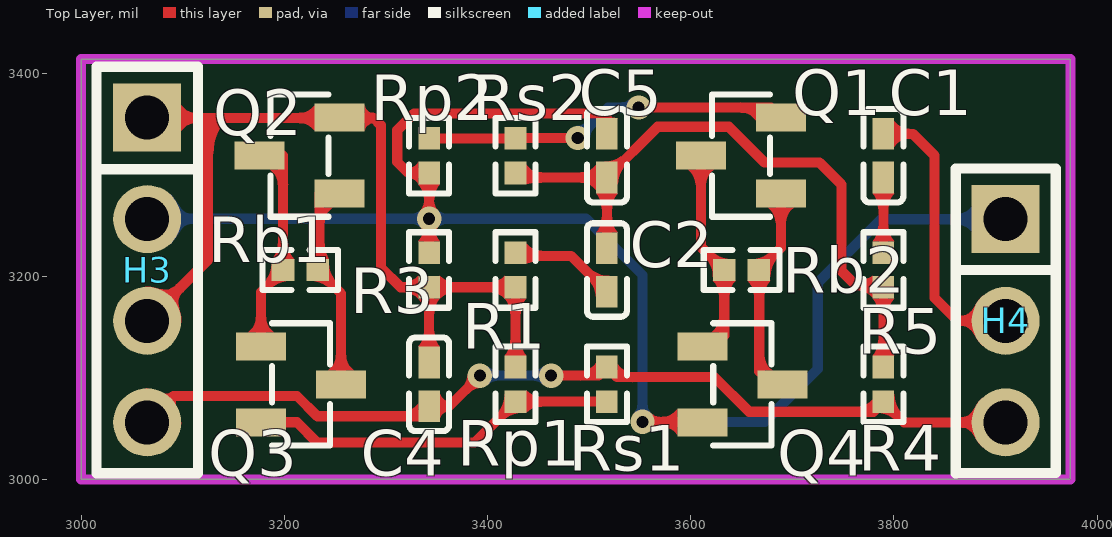
[diagram p0: Top Layer view]
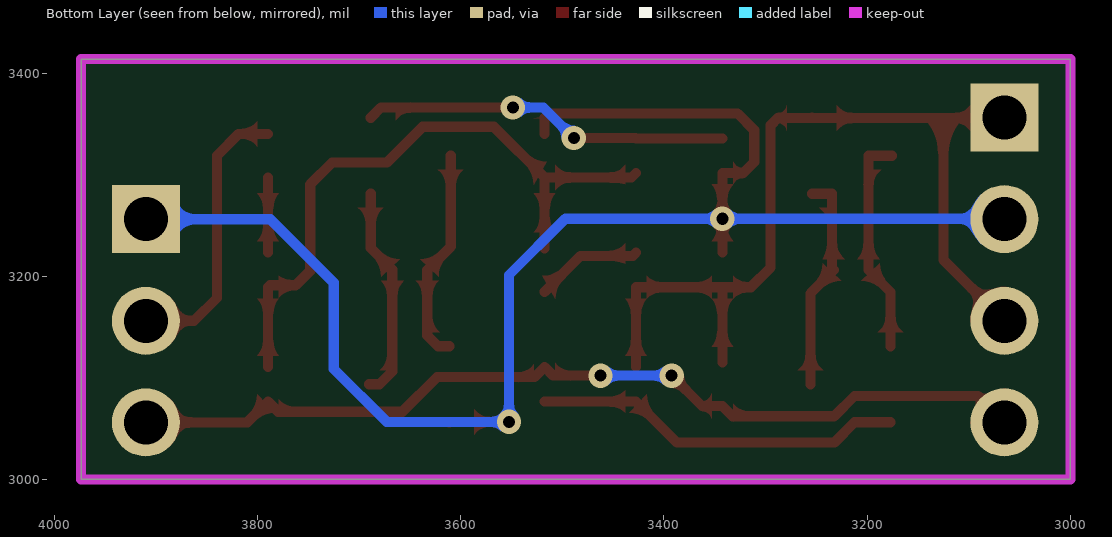
[diagram p1: Bottom Layer view, seen from below]
# Altium PCB MISC51661.pcbdoc
Units mil, origin at the board's own origin, x right, y up, seen from the top; angles counter-clockwise.
Board outline 973.64 x 413.7 mil, 2 copper layers (Top Layer, Bottom Layer), stack 62.206 mil thick; 20 components, 13 nets, 47 pads, 6 vias.

## Layer stack, top to bottom
Top Solder Mask Layer: solder mask 0.394, Dk 3.3
Top Layer: signal copper 1.379
Dielectric1: surface 59.449, FR4, Dk 4.5
Bottom Layer: signal copper 1.378
Bottom Solder Mask Layer: solder mask 0.394, Dk 3.3

## Board outline
3000,3413.7 3000,3000 3973.64,3000 3973.64,3413.7

## Design rules (kind name [scope] priority, off if disabled: settings)
BoardOutlineClearance copperThickness2oz_1 [All] p2 off: genericclearance=7.99 ignorepadtopadclearanceinfootprint=FALSE except(0: Arc-SplitContinuation Track-SplitContinuation SMDPad-SplitContinuation THPad-SplitContinuation Via-SplitContinuation Fill-SplitContinuation Region-SplitContinuation Poly-SplitContinuation Text-SplitContinuation Hole-SplitContinuation; 5.98: Arc-CutoutEdge Track-CutoutEdge SMDPad-CutoutEdge THPad-CutoutEdge Via-CutoutEdge Text-CutoutEdge; 6.9: Hole-OutlineEdge Hole-CutoutEdge; 10: Poly-OutlineEdge Poly-CutoutEdge; 11.81: Arc-OutlineEdge Track-OutlineEdge SMDPad-OutlineEdge THPad-OutlineEdge Via-OutlineEdge Fill-OutlineEdge Region-OutlineEdge Text-OutlineEdge Fill-CutoutEdge Region-CutoutEdge)
BoardOutlineClearance Plane_innerPlane_1 [All] p4 off: genericclearance=4.02 ignorepadtopadclearanceinfootprint=FALSE except(0: Arc-SplitContinuation Track-SplitContinuation SMDPad-SplitContinuation THPad-SplitContinuation Via-SplitContinuation Fill-SplitContinuation Region-SplitContinuation Poly-SplitContinuation Text-SplitContinuation Hole-SplitContinuation; 5.98: Arc-CutoutEdge Track-CutoutEdge SMDPad-CutoutEdge THPad-CutoutEdge Via-CutoutEdge Text-CutoutEdge; 6.9: Hole-OutlineEdge Hole-CutoutEdge; 10: Poly-OutlineEdge Poly-CutoutEdge; 11.81: Arc-OutlineEdge Track-OutlineEdge SMDPad-OutlineEdge THPad-OutlineEdge Via-OutlineEdge Fill-OutlineEdge Region-OutlineEdge Text-OutlineEdge Fill-CutoutEdge Region-CutoutEdge)
BoardOutlineClearance Copper_copperRegion_1 [All] p6 off: genericclearance=4.02 ignorepadtopadclearanceinfootprint=FALSE except(0: Arc-SplitContinuation Track-SplitContinuation SMDPad-SplitContinuation THPad-SplitContinuation Via-SplitContinuation Fill-SplitContinuation Region-SplitContinuation Poly-SplitContinuation Text-SplitContinuation Hole-SplitContinuation; 5.98: Arc-CutoutEdge Track-CutoutEdge SMDPad-CutoutEdge THPad-CutoutEdge Via-CutoutEdge Text-CutoutEdge; 6.9: Hole-OutlineEdge Hole-CutoutEdge; 10: Poly-OutlineEdge Poly-CutoutEdge; 11.81: Arc-OutlineEdge Track-OutlineEdge SMDPad-OutlineEdge THPad-OutlineEdge Via-OutlineEdge Fill-OutlineEdge Region-OutlineEdge Text-OutlineEdge Fill-CutoutEdge Region-CutoutEdge)
BoardOutlineClearance copperThickness1oz_1 [All] p8: genericclearance=4.02 ignorepadtopadclearanceinfootprint=FALSE except(0: Arc-SplitContinuation Track-SplitContinuation SMDPad-SplitContinuation THPad-SplitContinuation Via-SplitContinuation Fill-SplitContinuation Region-SplitContinuation Poly-SplitContinuation Text-SplitContinuation Hole-SplitContinuation; 5.98: Arc-CutoutEdge Track-CutoutEdge SMDPad-CutoutEdge THPad-CutoutEdge Via-CutoutEdge Text-CutoutEdge; 6.9: Hole-OutlineEdge Hole-CutoutEdge; 10: Poly-OutlineEdge Poly-CutoutEdge; 11.81: Arc-OutlineEdge Track-OutlineEdge SMDPad-OutlineEdge THPad-OutlineEdge Via-OutlineEdge Fill-OutlineEdge Region-OutlineEdge Text-OutlineEdge Fill-CutoutEdge Region-CutoutEdge)
Clearance copperThickness2oz [All] p1 off: gap=7.99 ignorepadtopadclearanceinfootprint=FALSE except(5.98: SMDPad-Track SMDPad-SMDPad THPad-Track SMDPad-THPad THPad-THPad Track-Via SMDPad-Via THPad-Via Via-Via Fill-SMDPad Region-SMDPad Fill-THPad Region-THPad Fill-Via Region-Via Fill-Fill Fill-Region Region-Region Arc-Track Arc-SMDPad Arc-THPad Arc-Via Fill-Arc Region-Arc Arc-Arc Text-Track SMDPad-Text Text-THPad Text-Via Fill-Text Region-Text Arc-Text Text-Text; 6.9: Hole-Track Hole-SMDPad Hole-THPad Hole-Via Fill-Hole Region-Hole Hole-Arc Hole-Text; 10: Poly-Track Poly-SMDPad Poly-THPad Poly-Via Poly-Fill Poly-Region Poly-Poly Poly-Arc Poly-Text Poly-Hole; 11.81: Fill-Track Region-Track)
Clearance Plane_innerPlane [All] p3 off: gap=4.02 ignorepadtopadclearanceinfootprint=FALSE except(5.98: SMDPad-Track SMDPad-SMDPad THPad-Track SMDPad-THPad THPad-THPad Track-Via SMDPad-Via THPad-Via Via-Via Fill-SMDPad Region-SMDPad Fill-THPad Region-THPad Fill-Via Region-Via Fill-Fill Fill-Region Region-Region Arc-Track Arc-SMDPad Arc-THPad Arc-Via Fill-Arc Region-Arc Arc-Arc Text-Track SMDPad-Text Text-THPad Text-Via Fill-Text Region-Text Arc-Text Text-Text; 6.9: Hole-Track Hole-SMDPad Hole-THPad Hole-Via Fill-Hole Region-Hole Hole-Arc Hole-Text; 10: Poly-Track Poly-SMDPad Poly-THPad Poly-Via Poly-Fill Poly-Region Poly-Poly Poly-Arc Poly-Text Poly-Hole; 11.81: Fill-Track Region-Track)
Clearance Copper_copperRegion [All] p5 off: gap=4.02 ignorepadtopadclearanceinfootprint=FALSE except(5.98: SMDPad-Track SMDPad-SMDPad THPad-Track SMDPad-THPad THPad-THPad Track-Via SMDPad-Via THPad-Via Via-Via Fill-SMDPad Region-SMDPad Fill-THPad Region-THPad Fill-Via Region-Via Fill-Fill Fill-Region Region-Region Arc-Track Arc-SMDPad Arc-THPad Arc-Via Fill-Arc Region-Arc Arc-Arc Text-Track SMDPad-Text Text-THPad Text-Via Fill-Text Region-Text Arc-Text Text-Text; 6.9: Hole-Track Hole-SMDPad Hole-THPad Hole-Via Fill-Hole Region-Hole Hole-Arc Hole-Text; 10: Poly-Track Poly-SMDPad Poly-THPad Poly-Via Poly-Fill Poly-Region Poly-Poly Poly-Arc Poly-Text Poly-Hole; 11.81: Fill-Track Region-Track)
Clearance copperThickness1oz [All] p7: gap=4.02 ignorepadtopadclearanceinfootprint=FALSE except(5.98: SMDPad-Track SMDPad-SMDPad THPad-Track SMDPad-THPad THPad-THPad Track-Via SMDPad-Via THPad-Via Via-Via Fill-SMDPad Region-SMDPad Fill-THPad Region-THPad Fill-Via Region-Via Fill-Fill Fill-Region Region-Region Arc-Track Arc-SMDPad Arc-THPad Arc-Via Fill-Arc Region-Arc Arc-Arc Text-Track SMDPad-Text Text-THPad Text-Via Fill-Text Region-Text Arc-Text Text-Text; 6.9: Hole-Track Hole-SMDPad Hole-THPad Hole-Via Fill-Hole Region-Hole Hole-Arc Hole-Text; 10: Poly-Track Poly-SMDPad Poly-THPad Poly-Via Poly-Fill Poly-Region Poly-Poly Poly-Arc Poly-Text Poly-Hole; 11.81: Fill-Track Region-Track)
DiffPairsRouting differentialPair [All] p1: maxlimit=6 minlimit=6 mostfreqgap=6 toplayer_minwidth=5 toplayer_prefwidth=10 toplayer_maxwidth=100 toplayer_mingap=6 toplayer_prefgap=6 toplayer_maxgap=6 bottomlayer_minwidth=5 bottomlayer_prefwidth=10 bottomlayer_maxwidth=100 bottomlayer_mingap=6 bottomlayer_prefgap=6 bottomlayer_maxgap=6 maxuncoupledlength=10
HoleToHoleClearance otherClearance [All] p1: gap=11.81 allowstackedmicrovias=TRUE
Length netLength [All] p1: minlimit=0 maxlimit=0
PasteMaskExpansion pasteMaskExpansion [All] p1: expansion=0
PlaneConnect innerPlane [All] p1: planeconnectstyle=Relief reliefexpansion=20 reliefentries=4 reliefconductorwidth=10 reliefairgap=10
PolygonConnect copperRegion [All] p1: connectstyle=Relief reliefconductorwidth=10 reliefentries=4 polygonreliefangle="90 Angle" airgapwidth=10 via.connectstyle=Relief via.reliefconductorwidth=10 via.reliefentries=4 via.polygonreliefangle="90 Angle" via.airgapwidth=10
RoutingVias viaSize [All] p1: holewidth=12.01 width=24.02 viastyle="Through Hole" minholewidth=11.81 minwidth=19.68 maxholewidth=248.03 maxwidth=393.7
SolderMaskExpansion solderMaskExpansion [IsVia] p1: expansion=-1000 istentingtop=TRUE
SolderMaskExpansion solderMaskExpansion [All] p2: expansion=2 istentingtop=FALSE
Width copperThickness2oz_2 [All] p1 off: maxlimit=100 minlimit=8 preferedwidth=10
Width copperThickness1oz_2 [All] p2: maxlimit=100 minlimit=5 preferedwidth=10

## Components (designator, comment, footprint, x,y, rotation, side; value= is the part's Value field where it differs from the comment)
C1 "0.1uF" C0402 3789.62,3318.7 r270 top
C2 "0.1uF" C0402 3517.5,3206.2 r270 top
C4 "0.1uF" C0402 3342.5,3093.7 r90 top
C5 "0.1uF" C0402 3517.5,3318.7 r90 top
H3 "" HDR-TH_4P-P2.54-V-M 3065,3206.2 r270 top
H4 "" HDR-TH_3P-P2.54-V-M 3910,3156.2 r270 top
Q1 "MMBT3906" SOT-23-3_L2.9-W1.3-P1.90-LS2.4-BR 3649.31,3318.7 r0 top
Q2 "MMBT3904" SOT-23-3_L2.9-W1.3-P1.90-LS2.4-BR 3215,3318.7 r0 top
Q3 "MMBT3906" SOT-23-3_L2.9-W1.3-P1.90-LS2.4-BR 3216.38,3093.7 r180 top
Q4 "MMBT3904" SOT-23-3_L2.9-W1.3-P1.90-LS2.4-BR 3650.69,3093.7 r180 top
R1 "1" R0402 3427.5,3206.2 r270 top
R3 "2.2K" R0402 3342.5,3206.2 r90 top
R4 "2.2K" R0402 3789.62,3093.7 r90 top
R5 "1" R0402 3789.62,3206.2 r270 top
Rb1 "1K" R0402 3215.69,3206.2 r180 top
Rb2 "1K" R0402 3650,3206.2 r0 top
Rp1 "200K" R0402 3427.5,3093.7 r90 top
Rp2 "200K" R0402 3342.5,3318.7 r270 top
Rs1 "200" R0402 3517.5,3093.7 r90 top
Rs2 "200" R0402 3427.5,3318.7 r270 top

## Footprints (in the part's own frame and the unit in brackets; to place one, negate y for a bottom-side part, rotate by r counter-clockwise, add the part's x,y. Pads: shape width x height; smd on the part's side, far side on the other; paste and mask are expansions set on the pad)
C0402 [mm]
  rect 0.79x0.54 smd paste-100 mask+0.051: 1(-0.545,0) 2(0.545,0)
  silkscreen extent -1.17,-0.5 1.17,0.5
HDR-TH_3P-P2.54-V-M [mm]
  rect 1.7x1.7 hole 1.1: 1(-2.54,0)
  round 1.7 hole 1.1: 2(0,0) 3(2.54,0)
  silkscreen extent -3.81,-1.25 3.81,1.25
HDR-TH_4P-P2.54-V-M [mm]
  rect 1.7x1.7 hole 1.1: 1(-3.81,0)
  round 1.7 hole 1.1: 2(-1.27,0) 3(1.27,0) 4(3.81,0)
  silkscreen extent -5.08,-1.27 5.08,1.27
R0402 [mm]
  rect 0.566x0.54 smd paste-100 mask+0.051: 1(-0.433,0) 2(0.433,0)
  silkscreen extent -0.94,-0.5 0.94,0.5
SOT-23-3_L2.9-W1.3-P1.90-LS2.4-BR [mm]
  rect 1.25x0.7 smd: 1(1,-0.95) 2(1,0.95) 3(-1,0)
  silkscreen extent -0.73,-1.53 0.73,1.53

## Via types
v1: diameter 24.02, hole 12, Top Layer to Bottom Layer, 6 vias

## Nets (pads, with @x,y where several pads share a name; then routed paths per layer and width w, separated by ;. In a path a pad name is that pad's centre, name@x,y a point inside that pad or via, vN(x,y) a via of type N, cw(c..) or ccw(c..) an arc to the next point about the centre after c; other vN are vias at no path point)
$1N718: Q2.3 Q3.1 Rb1.2 | length 219.6
  Top Layer w10: Q2.3 3198.65,3318.7 Rb1.2 3177.01,3184.56 Q3.1
$1N762: Q2.1 Q3.3 Rb1.1 | length 218.8
  Top Layer w10: Rb1.1 Rb1.1@3234.54,3204.39 ; Q2.1 3234.54,3281.3 Rb1.1@3234.54,3204.39 ; Q3.3 3255.75,3183.18 Rb1.1@3234.54,3204.39
$1N790: Q3.2 Rp1.1 Rs1.1 | length 365.5
  Top Layer w10: Q3.2 3212.4,3056.3 3232.4,3036.3 3387.14,3036.3 Rp1.1 Rs1.1
$1N794: C4.2 H3.1 H3.3 Q2.2 R1.2 R3.1 Rp1.2 | length 891
  Top Layer w10: H3.3 3125,3216.2 3125,3355.75 ; H3.1 3065.45,3355.75 3125,3355.75 ; Q2.2 Q2.2@3254.72,3355.75 ; C4.2 R3.1 ; Rp1.2 R1.2 R3.1 ; 3125,3355.75 Q2.2@3254.72,3355.75 ; Q2.2@3254.72,3355.75 3287.95,3355.75 3295,3348.7 3295,3208.7 3314.54,3189.16 R3.1
$1N871: C4.1 H3.4 H4.3 R4.1 Rs1.2 | length 915
  Top Layer w10: H3.4 3091.04,3082.24 3212.5,3082.24 3232.5,3062.24 3332.5,3062.24 C4.1 3362.5,3072.24 v1(3392.5,3102.24) ; v1(3462.5,3102.24) 3509,3102.24 Rs1.2 3527.5,3100.74 3623.42,3100.74 3657.5,3066.66 3779.62,3066.66 R4.1 3810.08,3056.2 H4.3
  Bottom Layer w10: v1(3392.5,3102.24) v1(3462.5,3102.24)
$1N1153: Q1.1 Q4.3 Rb2.2 | length 212.2
  Top Layer w10: Rb2.2 Rb2.2@3667.47,3206.63 ; Q1.1 3688.68,3227.84 Rb2.2@3667.47,3206.63 ; Q4.3 3680,3093.7 3667.47,3106.23 Rb2.2@3667.47,3206.63
$1N1158: Q1.3 Q4.1 Rb2.1 | length 212.6
  Top Layer w10: Q1.3 3609.94,3229.22 Rb2.1 3632.96,3141.66 3622.4,3131.1 Q4.1
$1N1162: Q1.2 Rp2.1 Rs2.1 | length 362.9
  Top Layer w10: Rp2.1 Rs2.1 3427.86,3336.1 v1(3488.68,3336.1) ; v1(3548.68,3366.1) 3678.68,3366.1 Q1.2
  Bottom Layer w10: v1(3488.68,3336.1) 3518.68,3366.1 v1(3548.68,3366.1)
$1N1224: C2.2 R1.1 | length 105.9
  Top Layer w10: R1.1 3430.64,3220.1 3482.14,3220.1 C2.2
$1N1967: C1.1 H4.2 | length 278.6
  Top Layer w10: C1.1 3818.54,3340.16 3840,3318.7 3840,3178.7 3862.5,3156.2 H4.2
$1N1970: C1.2 R5.1 | length 74
  Top Layer w10: R5.1 C1.2
$1N1975: C2.1 C5.1 R4.2 R5.2 Rs2.2 | length 647.9
  Top Layer w10: Rs2.2 3431.92,3297.24 C5.1 ; C2.1 C5.1 ; R4.2 R5.2 3787.6,3191.17 3762.53,3191.17 3748.21,3205.49 3748.21,3290.49 3726.82,3311.89 3672.86,3311.89 3637.5,3347.24 3567.5,3347.24 C5.1
$1N2087: C5.2 H3.2 H4.1 Q4.2 R3.2 Rp2.2 | length 1580.5
  Top Layer w10: R3.2 v1(3342.5,3256.66) Rp2.2 3322.04,3301.66 3311.16,3312.54 3311.16,3343.82 3327.5,3360.16 3513.54,3360.16 3517.5,3356.2 C5.2 ; v1(3552.5,3056.66) 3610.96,3056.66 Q4.2
  Bottom Layer w10: H3.2 3065.46,3256.66 v1(3342.5,3256.66) 3497.04,3256.66 3552.5,3201.2 v1(3552.5,3056.66) 3672.96,3056.66 3725,3108.7 3725,3193.7 3787.5,3256.2 H4.1

## Keep-outs
Board Outline Layer:
  the board outline again, w10

## Other copper
Top Layer:
  region net $1N794: 3337.5,3145.71 3347.5,3145.71 3347.87,3141.64 3348.95,3137.7 3350.73,3134.02 3353.13,3130.71 3331.87,3130.71 3334.27,3134.02 3336.05,3137.7 3337.13,3141.64 3337.5,3145.71
  region net $1N871: 3362.5,3077.24 3362.5,3067.24 3359.94,3066.89 3357.56,3065.87 3355.54,3064.26 3354.03,3062.16 3353.13,3059.74 3353.13,3084.74 3354.03,3082.32 3355.54,3080.22 3357.56,3078.61 3359.94,3077.59
  region net $1N871: 3316.87,3057.24 3316.87,3067.24 3320.33,3067.56 3323.67,3068.52 3326.77,3070.07 3329.54,3072.17 3331.87,3074.74 3331.87,3056.69 3324.38,3057.1 3316.87,3057.24
  region net $1N2087: 3512.5,3356.2 3522.5,3356.2 3525.3,3355.84 3528.13,3355.71 3506.87,3355.71 3509.7,3355.84 3512.5,3356.2
  region net $1N1975: 3522.5,3266.69 3512.5,3266.69 3512.13,3270.76 3511.05,3274.7 3509.27,3278.38 3506.87,3281.69 3528.13,3281.69 3525.73,3278.38 3523.95,3274.7 3522.87,3270.76 3522.5,3266.69
  region net $1N1975: 3491.87,3292.24 3491.87,3302.24 3495.33,3302.56 3498.67,3303.52 3501.77,3305.07 3504.54,3307.17 3506.87,3309.74 3506.87,3284.74 3504.54,3287.31 3501.77,3289.41 3498.67,3290.97 3495.33,3291.92 3491.87,3292.24
  region net $1N1975: 3531.29,3318.1 3533.43,3306.1 3531.16,3302.5 3529.49,3298.58 3528.47,3294.44 3528.13,3290.19 3515.38,3312.79 3519.62,3313.14 3523.76,3314.15 3527.68,3315.82 3531.29,3318.1
  region net $1N1224: 3501.57,3193.6 3503.71,3205.6 3507.32,3203.32 3511.24,3201.65 3515.38,3200.64 3519.62,3200.29 3506.87,3177.69 3506.53,3181.94 3505.51,3186.08 3503.84,3190 3501.57,3193.6
  region net $1N1975: 3512.5,3258.21 3522.5,3258.21 3522.87,3254.14 3523.95,3250.2 3525.73,3246.52 3528.13,3243.21 3506.87,3243.21 3509.27,3246.52 3511.05,3250.2 3512.13,3254.14 3512.5,3258.21
  region net $1N1970: 3794.62,3266.69 3784.62,3266.69 3784.25,3270.76 3783.16,3274.7 3781.39,3278.38 3778.99,3281.69 3800.25,3281.69 3797.85,3278.38 3796.07,3274.7 3794.98,3270.76 3794.62,3266.69
  region net $1N1967: 3815.25,3345.16 3815.25,3335.16 3811.79,3334.84 3808.45,3333.89 3805.35,3332.33 3802.58,3330.23 3800.25,3327.66 3800.25,3352.66 3802.58,3350.09 3805.35,3347.99 3808.45,3346.44 3811.79,3345.48 3815.25,3345.16
  region net $1N1967: 3864.27,3151.2 3864.27,3161.2 3866.87,3161.32 3869.11,3161.65 3871.03,3162.19 3872.67,3162.91 3874.08,3163.82 3875.31,3164.88 3876.4,3166.09 3877.41,3167.43 3879.32,3170.45 3881.43,3173.82 3884.1,3177.42 3885.75,3179.28 3887.69,3181.14 3887.69,3131.26 3885.75,3133.13 3884.1,3134.98 3881.43,3138.58 3879.32,3141.95 3877.41,3144.97 3876.4,3146.31 3875.31,3147.52 3874.08,3148.58 3872.67,3149.49 3871.03,3150.21 3869.11,3150.75 3866.87,3151.09
  region net $1N871: 3864.27,3051.2 3864.27,3061.2 3866.87,3061.32 3869.11,3061.65 3871.03,3062.19 3872.67,3062.91 3874.08,3063.82 3875.31,3064.88 3876.4,3066.09 3877.41,3067.43 3879.32,3070.45 3881.43,3073.82 3884.1,3077.42 3885.75,3079.28 3887.69,3081.14 3887.69,3031.26 3885.75,3033.13 3884.1,3034.98 3881.43,3038.58 3879.32,3041.95 3877.41,3044.97 3876.4,3046.31 3875.31,3047.52 3874.08,3048.58 3872.67,3049.49 3871.03,3050.21 3869.11,3050.75 3866.87,3051.09
  region net $1N718: 3172.01,3159.88 3182.01,3159.88 3182.33,3156.42 3183.29,3153.08 3184.84,3149.98 3186.94,3147.21 3189.51,3144.88 3164.51,3144.88 3167.08,3147.21 3169.18,3149.98 3170.74,3153.08 3171.69,3156.42 3172.01,3159.88
  region net $1N762: 3250.75,3122.48 3260.75,3122.48 3261.07,3119.02 3262.03,3115.68 3263.58,3112.58 3265.68,3109.81 3268.25,3107.48 3243.25,3107.48 3245.82,3109.81 3247.92,3112.58 3249.48,3115.68 3250.43,3119.02 3250.75,3122.48
  region net $1N762: 3239.54,3252.52 3229.54,3252.52 3229.71,3260.02 3229.76,3267.52 3247.04,3267.52 3244.46,3265.19 3242.37,3262.42 3240.81,3259.32 3239.86,3255.98 3239.54,3252.52
  region net $1N794: 3214.76,3350.75 3214.76,3360.75 3218.22,3361.07 3221.56,3362.03 3224.67,3363.58 3227.43,3365.68 3229.76,3368.25 3229.76,3343.25 3227.43,3345.83 3224.67,3347.92 3221.56,3349.48 3218.22,3350.43 3214.76,3350.75
  region net $1N794: 3287.95,3360.75 3287.95,3350.75 3285.44,3350.4 3283.13,3349.37 3281.19,3347.75 3279.77,3345.66 3278.98,3343.25 3278.98,3368.25 3279.77,3365.85 3281.19,3363.75 3283.13,3362.13 3285.44,3361.1 3287.95,3360.75
  region net $1N718: 3203.65,3289.92 3193.65,3289.92 3193.33,3293.38 3192.38,3296.72 3190.82,3299.82 3188.72,3302.59 3186.15,3304.92 3200.24,3304.92 3200.62,3299.77 3201.77,3294.73 3203.65,3289.92
  region net $1N1153: 3693.68,3252.52 3683.68,3252.52 3683.36,3255.98 3682.4,3259.32 3680.85,3262.42 3678.75,3265.19 3676.18,3267.52 3701.18,3267.52 3698.61,3265.19 3696.51,3262.42 3694.95,3259.32 3694,3255.98 3693.68,3252.52
  region net $1N1162: 3649.07,3361.1 3649.07,3371.1 3656.55,3370.19 3664.07,3369.88 3664.07,3353.6 3661.74,3356.17 3658.98,3358.27 3655.87,3359.83 3652.53,3360.78 3649.07,3361.1
  region net $1N1158: 3614.94,3289.92 3604.94,3289.92 3604.62,3293.38 3603.66,3296.72 3602.11,3299.82 3600.01,3302.59 3597.44,3304.92 3622.44,3304.92 3619.87,3302.59 3617.77,3299.82 3616.21,3296.72 3615.26,3293.38 3614.94,3289.92
  region net $1N1158: 3627.96,3159.88 3637.96,3159.88 3636.83,3154.95 3636.15,3149.93 3635.93,3144.88 3620.46,3144.88 3623.03,3147.21 3625.13,3149.98 3626.68,3153.08 3627.64,3156.42 3627.96,3159.88
  region net $1N2087: 3571.71,3051.66 3571.71,3061.66 3575.17,3061.98 3578.51,3062.94 3581.62,3064.49 3584.38,3066.59 3586.71,3069.16 3586.71,3044.16 3584.38,3046.73 3581.62,3048.83 3578.51,3050.39 3575.17,3051.34 3571.71,3051.66
  region net $1N1153: 3662.47,3122.48 3672.47,3122.48 3672.79,3119.02 3673.74,3115.68 3675.29,3112.58 3677.39,3109.81 3679.97,3107.48 3665.45,3107.48 3665.12,3112.6 3664.12,3117.63 3662.47,3122.48
  region net $1N2087: 3337.5,3249.38 3347.5,3249.38 3347.87,3245.3 3348.95,3241.36 3350.73,3237.68 3353.13,3234.38 3331.87,3234.38 3334.27,3237.68 3336.05,3241.36 3337.13,3245.3 3337.5,3249.38
  region net $1N794: 3347.5,3163.03 3337.5,3163.03 3337.13,3167.1 3336.05,3171.04 3334.27,3174.72 3331.87,3178.03 3353.13,3178.03 3350.73,3174.72 3348.95,3171.04 3347.87,3167.1 3347.5,3163.03
  region net $1N794: 3316.87,3184.16 3316.87,3194.16 3320.18,3194.42 3323.41,3195.18 3326.49,3196.44 3329.33,3198.16 3331.87,3200.3 3331.87,3178.03 3329.33,3180.16 3326.49,3181.88 3323.41,3183.14 3320.18,3183.9 3316.87,3184.16
  region net $1N794: 3368.13,3194.16 3368.13,3184.16 3364.82,3183.9 3361.59,3183.14 3358.51,3181.88 3355.67,3180.16 3353.13,3178.03 3353.13,3200.3 3355.67,3198.16 3358.51,3196.44 3361.59,3195.18 3364.82,3194.42 3368.13,3194.16
  region net $1N1975: 3784.62,3136.88 3794.62,3136.88 3794.98,3132.8 3796.07,3128.86 3797.85,3125.18 3800.25,3121.88 3778.99,3121.88 3781.39,3125.18 3783.16,3128.86 3784.25,3132.8 3784.62,3136.88
  region net $1N871: 3763.99,3061.66 3763.99,3071.66 3767.45,3071.98 3770.78,3072.94 3773.89,3074.49 3776.66,3076.59 3778.99,3079.16 3778.99,3065.53 3775.08,3065.28 3771.24,3064.54 3767.52,3063.33 3763.99,3061.66
  region net $1N871: 3805.55,3067.8 3798.99,3060.22 3795.38,3062.5 3791.46,3064.17 3787.32,3065.18 3783.08,3065.53 3800.25,3083.71 3800.59,3079.46 3801.61,3075.32 3803.28,3071.4 3805.55,3067.8
  region net $1N718: 3193.65,3231.83 3203.65,3231.83 3203.91,3228.52 3204.67,3225.29 3205.93,3222.22 3207.65,3219.37 3209.79,3216.83 3187.52,3216.83 3189.65,3219.37 3191.37,3222.22 3192.63,3225.29 3193.39,3228.52 3193.65,3231.83
  region net $1N718: 3189.79,3190.27 3182.21,3196.83 3184.49,3200.44 3186.15,3204.36 3187.17,3208.5 3187.52,3212.74 3205.7,3195.57 3201.45,3195.23 3197.31,3194.21 3193.39,3192.54 3189.79,3190.27
  region net $1N762: 3229.54,3231.83 3239.54,3231.83 3239.81,3227.89 3240.64,3224.02 3242,3220.31 3243.87,3216.83 3222.04,3216.83 3224.61,3219.16 3226.71,3221.93 3228.26,3225.03 3229.22,3228.37 3229.54,3231.83
  region net $1N762: 3249.17,3196.83 3241.59,3190.27 3237.99,3192.54 3234.07,3194.21 3229.93,3195.23 3225.68,3195.57 3243.87,3212.74 3244.21,3208.5 3245.23,3204.36 3246.89,3200.44 3249.17,3196.83
  region net $1N794: 3432.5,3163.03 3422.5,3163.03 3422.13,3167.1 3421.05,3171.04 3419.27,3174.72 3416.87,3178.03 3438.13,3178.03 3435.73,3174.72 3433.95,3171.04 3432.87,3167.1 3432.5,3163.03
  region net $1N794: 3401.87,3184.16 3401.87,3194.16 3405.18,3194.42 3408.41,3195.18 3411.49,3196.44 3414.33,3198.16 3416.87,3200.3 3416.87,3178.03 3414.33,3180.16 3411.49,3181.88 3408.41,3183.14 3405.18,3183.9 3401.87,3184.16
  region net $1N1224: 3453.13,3225.1 3453.13,3215.1 3448.01,3214.76 3442.98,3213.76 3438.13,3212.11 3438.13,3232.6 3440.46,3230.02 3443.23,3227.92 3446.33,3226.37 3449.67,3225.42 3453.13,3225.1
  region net $1N1153: 3672.47,3180.57 3662.47,3180.57 3662.19,3183.92 3661.37,3187.19 3660.02,3190.27 3658.18,3193.09 3655.91,3195.57 3678.18,3195.57 3675.74,3192.28 3673.94,3188.6 3672.84,3184.65 3672.47,3180.57
  region net $1N1153: 3675.9,3222.13 3683.48,3215.57 3681.2,3211.96 3679.54,3208.04 3678.52,3203.91 3678.18,3199.66 3659.99,3216.83 3664.24,3217.17 3668.38,3218.19 3672.3,3219.86 3675.9,3222.13
  region net $1N1158: 3616.52,3215.57 3624.1,3222.13 3627.7,3219.86 3631.62,3218.19 3635.76,3217.17 3640.01,3216.83 3621.82,3199.66 3621.48,3203.91 3620.46,3208.04 3618.8,3211.96 3616.52,3215.57
  region net $1N1158: 3637.96,3180.57 3627.96,3180.57 3627.7,3183.88 3626.94,3187.11 3625.68,3190.19 3623.96,3193.03 3621.82,3195.57 3644.09,3195.57 3641.96,3193.03 3640.24,3190.19 3638.98,3187.11 3638.22,3183.88 3637.96,3180.57
  region net $1N1975: 3763.99,3186.17 3763.99,3196.17 3767.91,3196.44 3771.77,3197.22 3775.48,3198.52 3778.99,3200.3 3778.99,3178.67 3776.66,3181.25 3773.89,3183.35 3770.78,3184.9 3767.45,3185.85 3763.99,3186.17
  region net $1N1975: 3794.62,3163.03 3784.62,3163.03 3784.25,3167.1 3783.16,3171.04 3781.39,3174.72 3778.99,3178.03 3800.25,3178.03 3797.85,3174.72 3796.07,3171.04 3794.98,3167.1 3794.62,3163.03
  region net $1N1970: 3784.62,3249.38 3794.62,3249.38 3794.98,3245.3 3796.07,3241.36 3797.85,3237.68 3800.25,3234.38 3778.99,3234.38 3781.39,3237.68 3783.16,3241.36 3784.25,3245.3 3784.62,3249.38
  region net $1N794: 3422.5,3136.88 3432.5,3136.88 3432.87,3132.8 3433.95,3128.86 3435.73,3125.18 3438.13,3121.88 3416.87,3121.88 3419.27,3125.18 3421.05,3128.86 3422.13,3132.8 3422.5,3136.88
  region net $1N790: 3453.13,3081.66 3453.13,3071.66 3449.82,3071.4 3446.59,3070.64 3443.51,3069.38 3440.67,3067.66 3438.13,3065.53 3438.13,3087.8 3440.67,3085.66 3443.51,3083.94 3446.59,3082.68 3449.82,3081.92 3453.13,3081.66
  region net $1N790: 3418.13,3060.22 3411.57,3067.8 3413.84,3071.4 3415.51,3075.32 3416.53,3079.46 3416.87,3083.71 3434.04,3065.53 3429.8,3065.18 3425.66,3064.17 3421.74,3062.5 3418.13,3060.22
  region net $1N2087: 3322.04,3296.66 3322.04,3306.66 3324.46,3306.93 3326.76,3307.73 3328.83,3309.02 3330.56,3310.74 3331.87,3312.8 3331.87,3290.53 3330.56,3292.58 3328.83,3294.3 3326.76,3295.59 3324.46,3296.39 3322.04,3296.66
  region net $1N2087: 3347.5,3275.53 3337.5,3275.53 3337.13,3279.6 3336.05,3283.54 3334.27,3287.22 3331.87,3290.53 3353.13,3290.53 3350.73,3287.22 3348.95,3283.54 3347.87,3279.6 3347.5,3275.53
  region net $1N871: 3543.13,3105.74 3543.13,3095.74 3539.59,3097.41 3535.88,3098.62 3532.03,3099.36 3528.13,3099.61 3528.13,3113.24 3530.46,3110.67 3533.23,3108.57 3536.33,3107.02 3539.67,3106.06 3543.13,3105.74
  region net $1N871: 3491.87,3097.24 3491.87,3107.24 3495.33,3107.56 3498.67,3108.52 3501.77,3110.07 3504.54,3112.17 3506.87,3114.74 3506.87,3099.61 3501.8,3099.34 3496.78,3098.55 3491.87,3097.24
  region net $1N1975: 3453.13,3302.24 3453.13,3292.24 3448.09,3292.05 3443.08,3291.48 3438.13,3290.53 3438.13,3309.74 3440.46,3307.17 3443.23,3305.07 3446.33,3303.52 3449.67,3302.56 3453.13,3302.24
  region net $1N794: 3113.46,3360.75 3113.46,3350.75 3110.01,3350.43 3106.67,3349.48 3103.56,3347.92 3100.8,3345.83 3098.46,3343.25 3098.46,3368.25 3100.8,3365.68 3103.56,3363.58 3106.67,3362.03 3110.01,3361.07 3113.46,3360.75
  region net $1N794: 3093.8,3192.08 3100.87,3185 3099.11,3183.08 3097.77,3181.26 3096.79,3179.53 3096.15,3177.85 3095.78,3176.21 3095.67,3174.59 3095.75,3172.96 3095.99,3171.31 3096.77,3167.82 3097.66,3163.94 3098.32,3159.51 3098.46,3157.03 3098.41,3154.34 3063.14,3189.61 3065.83,3189.66 3068.31,3189.52 3072.74,3188.86 3076.61,3187.97 3080.11,3187.19 3081.76,3186.95 3083.39,3186.87 3085.01,3186.99 3086.65,3187.35 3088.33,3187.99 3090.06,3188.97 3091.88,3190.31
  region net $1N871: 3087.5,3085.78 3094.58,3078.71 3093.75,3077.64 3093.24,3076.45 3093,3075.13 3093,3073.72 3093.21,3072.21 3093.58,3070.64 3094.67,3067.34 3097.24,3060.55 3098.15,3057.31 3098.38,3055.78 3098.41,3054.34 3063.14,3089.61 3064.58,3089.58 3066.11,3089.35 3069.35,3088.45 3076.14,3085.87 3079.44,3084.78 3081.01,3084.41 3082.52,3084.2 3083.93,3084.2 3085.25,3084.44 3086.44,3084.95
  region net $1N2087: 3347.5,3240.25 3337.5,3240.25 3337.41,3241.37 3337.16,3242.5 3336.27,3244.74 3335,3246.83 3333.55,3248.66 3351.45,3248.66 3350,3246.83 3348.73,3244.74 3347.84,3242.5 3347.59,3241.37
  region net $1N2087: 3337.5,3273.07 3347.5,3273.07 3347.59,3271.95 3347.84,3270.82 3348.73,3268.59 3350,3266.49 3351.45,3264.67 3333.55,3264.67 3335,3266.49 3336.27,3268.59 3337.16,3270.82 3337.41,3271.95
  region net $1N2087: 3568.91,3061.66 3568.91,3051.66 3567.79,3051.57 3566.66,3051.32 3564.43,3050.43 3562.33,3049.16 3560.51,3047.71 3560.51,3065.61 3562.33,3064.16 3564.43,3062.9 3566.66,3062 3567.79,3061.75
  region net $1N871: 3384.43,3087.1 3377.36,3094.17 3378.09,3095.03 3378.71,3096.01 3379.66,3098.22 3380.24,3100.59 3380.51,3102.91 3393.17,3090.25 3390.85,3089.98 3388.48,3089.4 3386.26,3088.45 3385.29,3087.83
  region net $1N794: 3130,3320.75 3130.29,3326.1 3131.15,3331.4 3132.57,3336.56 3134.53,3341.55 3137.02,3346.3 3140,3350.75 3125,3355.75 3110,3350.75 3112.98,3346.3 3115.47,3341.55 3117.43,3336.56 3118.85,3331.4 3119.71,3326.1 3120,3320.75 3130,3320.75
Bottom Layer:
  region net $1N2087: 3861.54,3251.2 3861.54,3261.2 3864.99,3261.52 3868.33,3262.48 3871.44,3264.03 3874.2,3266.13 3876.54,3268.7 3876.54,3243.7 3874.2,3246.27 3871.44,3248.37 3868.33,3249.93 3864.99,3250.88 3861.54,3251.2
  region net $1N2087: 3110.39,3261.66 3111.08,3251.66 3108.49,3251.55 3106.26,3251.21 3104.34,3250.67 3102.69,3249.93 3101.27,3249.02 3100.02,3247.95 3098.91,3246.73 3097.89,3245.38 3095.95,3242.34 3093.83,3238.95 3091.19,3235.31 3089.55,3233.45 3087.65,3231.57 3086.96,3281.45 3088.94,3279.6 3090.62,3277.76 3093.3,3274.18 3097.29,3267.84 3098.28,3266.51 3099.35,3265.31 3100.57,3264.26 3101.97,3263.36 3103.61,3262.64 3105.52,3262.11 3107.77,3261.77
  region net $1N1162: 3532.27,3361.1 3532.27,3371.1 3533.39,3371.19 3534.52,3371.44 3536.75,3372.34 3538.85,3373.6 3540.67,3375.05 3540.67,3357.15 3538.85,3358.6 3536.75,3359.87 3534.52,3360.76 3533.39,3361.01
  region net $1N1162: 3496.75,3351.24 3503.82,3344.17 3503.09,3343.31 3502.47,3342.34 3501.52,3340.12 3500.94,3337.75 3500.67,3335.43 3488.01,3348.09 3490.33,3348.36 3492.7,3348.94 3494.92,3349.89 3495.89,3350.51
  region net $1N2087: 3326.09,3251.66 3326.09,3261.66 3327.21,3261.75 3328.34,3262 3330.57,3262.9 3332.67,3264.16 3334.49,3265.61 3334.49,3247.71 3332.67,3249.16 3330.57,3250.43 3328.34,3251.32 3327.21,3251.57
  region net $1N2087: 3358.91,3261.66 3358.91,3251.66 3357.79,3251.57 3356.66,3251.32 3354.43,3250.43 3352.33,3249.16 3350.51,3247.71 3350.51,3265.61 3352.33,3264.16 3354.43,3262.9 3356.66,3262 3357.79,3261.75
  region net $1N2087: 3547.5,3073.07 3557.5,3073.07 3557.59,3071.95 3557.84,3070.82 3558.73,3068.59 3560,3066.49 3561.45,3064.67 3543.55,3064.67 3545,3066.49 3546.27,3068.59 3547.16,3070.82 3547.41,3071.95
  region net $1N2087: 3568.91,3061.66 3568.91,3051.66 3567.79,3051.57 3566.66,3051.32 3564.43,3050.43 3562.33,3049.16 3560.51,3047.71 3560.51,3065.61 3562.33,3064.16 3564.43,3062.9 3566.66,3062 3567.79,3061.75
  region net $1N871: 3408.91,3107.24 3408.91,3097.24 3407.79,3097.15 3406.66,3096.9 3404.43,3096.01 3402.33,3094.74 3400.51,3093.29 3400.51,3111.19 3402.33,3109.74 3404.43,3108.48 3406.66,3107.58 3407.79,3107.33
  region net $1N871: 3446.09,3097.24 3446.09,3107.24 3447.21,3107.33 3448.34,3107.58 3450.57,3108.48 3452.67,3109.74 3454.49,3111.19 3454.49,3093.29 3452.67,3094.74 3450.57,3096.01 3448.34,3096.9 3447.21,3097.15